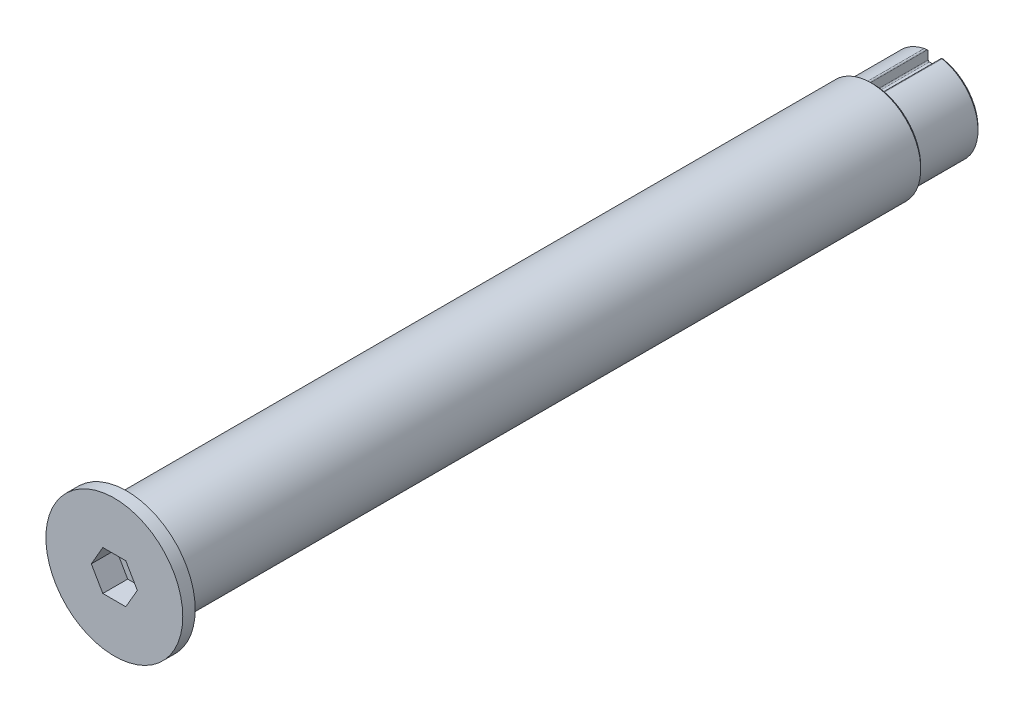
SolidWorks part; units mm, degrees
material "42CrMo"
ref_plane "前视基准面" through (0, 0, 0) normal (0, 0, 1) x (1, 0, 0)
ref_plane "上视基准面" through (0, 0, 0) normal (0, 1, 0) x (1, 0, 0)
ref_plane "右视基准面" through (0, 0, 0) normal (1, 0, 0) x (0, 0, -1)
sketch "草图1" plane through (0, 0, 0) normal (0, 0, 1) x (1, 0, 0)
  circle A0 centre (0, 0) radius 20
  dimension "D1" = 40
extrude "凸台-拉伸1" add sketch "草图1" along normal blind 325
sketch "草图2" plane through (0, 0, 325) normal (0, 0, 1) x (1, 0, 0)
  circle A0 centre (0, 0) radius 27.5
  dimension "D1" = 55
extrude "凸台-拉伸2" add sketch "草图2" along normal blind 5
sketch "草图3" plane through (0, 0, 330) normal (0, 0, 1) x (1, 0, 0)
  line L1 (9.2376, 0) -> (4.6188, 8)
  line L2 (4.6188, 8) -> (-4.6188, 8)
  line L3 (-4.6188, 8) -> (-9.2376, 0)
  line L4 (-9.2376, 0) -> (-4.6188, -8)
  line L5 (-4.6188, -8) -> (4.6188, -8)
  line L6 (4.6188, -8) -> (9.2376, 0)
  circle A0 centre (0, 0) radius 8 construction
  dimension "D1" = 16
extrude "切除-拉伸1" cut sketch "草图3" against normal blind 10
sketch "草图4" plane through (0, 0, 0) normal (0, 0, -1) x (-1, 0, 0)
  circle A0 centre (0, 0) radius 18
  dimension "D1" = 36
extrude "切除-拉伸2" cut sketch "草图4" against normal blind 25 flip side to cut
cosmetic thread "装饰螺纹线2" parameters "D2"=15
chamfer "倒角1" distance 1 angle 45 1 edges at (-20, 0, 25)
chamfer "倒角2" distance 1 angle 45 1 edges at (-18, 0, 0)
fillet "圆角1" radius 0.5 1 edges at (20, 0, 325)
sketch "草图5" plane through (0, 0, 0) normal (0, 0, -1) x (-1, 0, 0)
  line L0 (0, 0) -> (0, 18) construction
  line L2 (-3, 23) -> (3, 23)
  line L3 (-3, 23) -> (-3, 13)
  line L4 (-3, 13) -> (3, 13)
  line L5 (3, 23) -> (3, 13)
  line L6 (-3, 23) -> (3, 13) construction
  line L7 (-3, 13) -> (3, 23) construction
  circle A1 centre (0, 0) radius 18 construction
  point P10 (0, 18)
  dimension "D1" = 6
  dimension "D2" = 5
extrude "切除-拉伸3" cut sketch "草图5" against normal up to surface (25 mm away) up to face at (-19, 0, 25)
fillet "圆角2" radius 0.5 4 edges at (-3, 13, 12.5) (3, 13, 12.5) (3, 17.7482, 13) (-3, 17.7482, 13)
